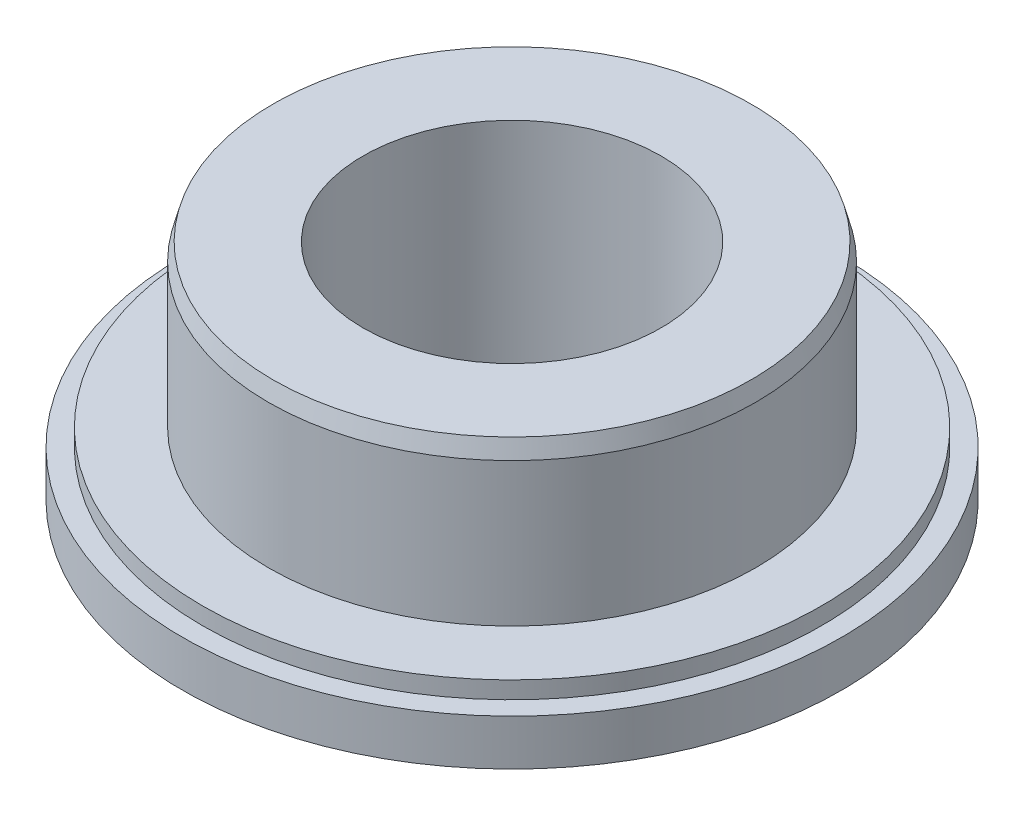
from build123d import *

# Parameters (mm, degrees)
CHAMFER1_SIZE  = 3
CHAMFER1_SIZE2 = 0.803847577


with BuildPart() as part:
    # Sketch1 → Revolve1 (revolve)
    with BuildSketch(Plane.XY, mode=Mode.PRIVATE) as revolve1_sk:
        Polygon((26, 31), (42.5, 31), (42.5, 3), (54, 3), (54, 0), (57.5, 0), (57.5, -8), (26, -8), align=None)
    revolve(revolve1_sk.sketch.rotate(Axis((0, 0, 0), (0, 1, 0)), 90), axis=Axis((0, 0, 0), (0, 1, 0)))

    # Chamfer1
    chamfer1_edges = [part.edges().sort_by_distance(p)[0] for p in [
        (0, 31, 42.5),
    ]]
    chamfer1_side = [part.faces().sort_by_distance(p)[0] for p in [
        (0, 17, 42.5),
    ]]
    chamfer(chamfer1_edges, length=CHAMFER1_SIZE, length2=CHAMFER1_SIZE2, reference=chamfer1_side[0])


solid = part.part
